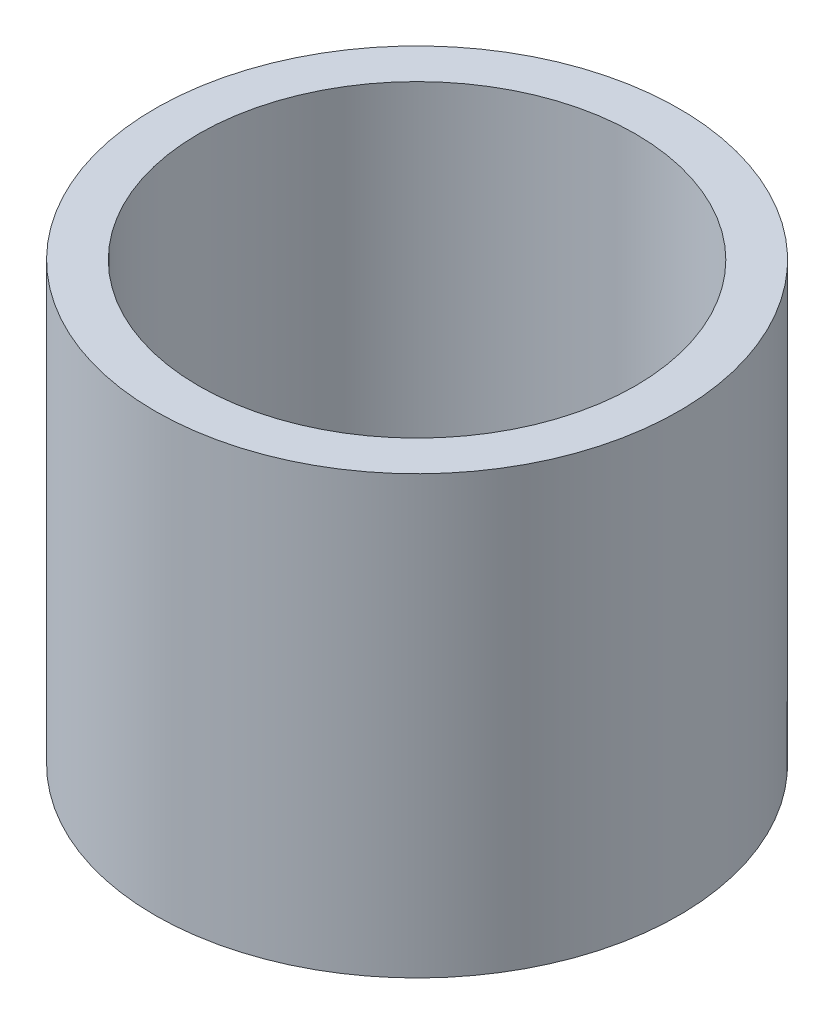
from build123d import *

# Parameters (mm, degrees)
SKETCH1_R           = 3
SKETCH1_R_2         = 2.5
BOSS_EXTRUDE1_DEPTH = 5


with BuildPart() as part:
    # Sketch1 → Boss-Extrude1 (new body)
    with BuildSketch(Plane(origin=(0, 0, 0), x_dir=(1, 0, 0), z_dir=(0, 1, 0))):
        with Locations(Location((0, 0, 0), (0, 0, 270))):
            Circle(SKETCH1_R)
        with Locations(Location((0, 0, 0), (0, 0, 270))):
            Circle(SKETCH1_R_2, mode=Mode.SUBTRACT)
    extrude(amount=BOSS_EXTRUDE1_DEPTH)


solid = part.part
